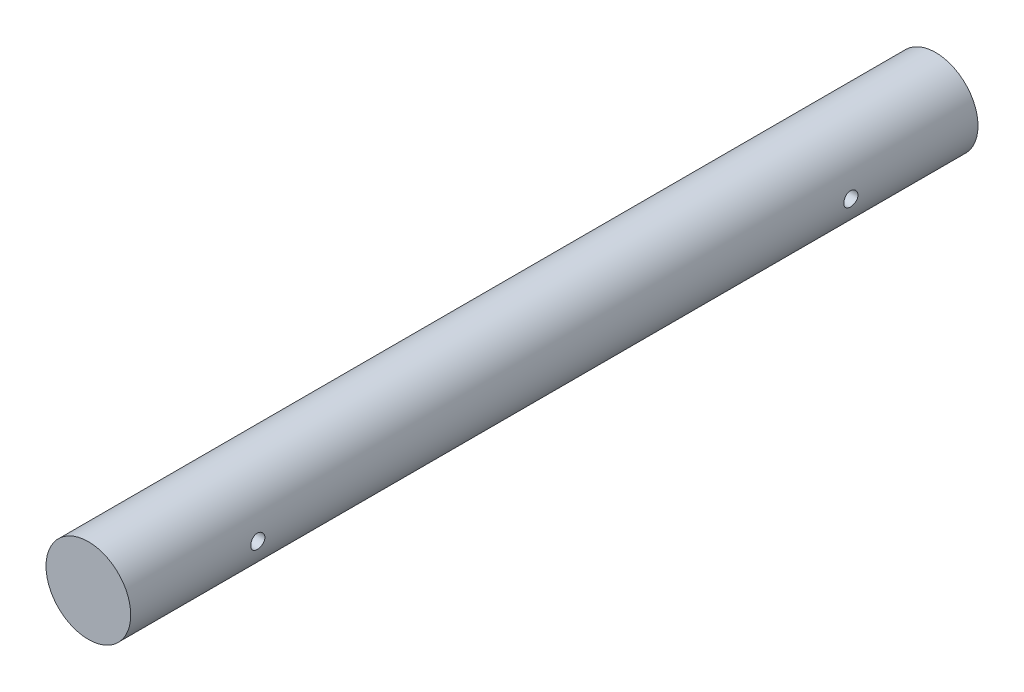
from build123d import *

# Parameters (mm, degrees)
BOSS_EXTRUDE1_DEPTH      = 60
BOSS_EXTRUDE1_DEPTH_BACK = 60
SKETCH1_R                = 6
CUT_EXTRUDE1_DEPTH       = 99.037186822
CUT_EXTRUDE1_DEPTH_BACK  = 99.037186822
SKETCH2_R                = 1


with BuildPart() as part:
    # Sketch1 → Boss-Extrude1 (new, two sides: drawn at the far end of the back side and taken through both)
    with BuildSketch(Plane.XY.offset(-BOSS_EXTRUDE1_DEPTH_BACK)):
        with Locations((-100, 71.3)):
            Circle(SKETCH1_R)
    extrude(amount=BOSS_EXTRUDE1_DEPTH + BOSS_EXTRUDE1_DEPTH_BACK)

    # Sketch2 → Cut-Extrude1 (cut, two sides: drawn at the far end of the back side and taken through both)
    with BuildSketch(Plane.ZY.offset(100).offset(-CUT_EXTRUDE1_DEPTH_BACK)):
        with Locations((-42, 71.3)):
            Circle(SKETCH2_R)
        with Locations((42, 71.3)):
            Circle(SKETCH2_R)
    extrude(amount=CUT_EXTRUDE1_DEPTH + CUT_EXTRUDE1_DEPTH_BACK, mode=Mode.SUBTRACT)


solid = part.part
